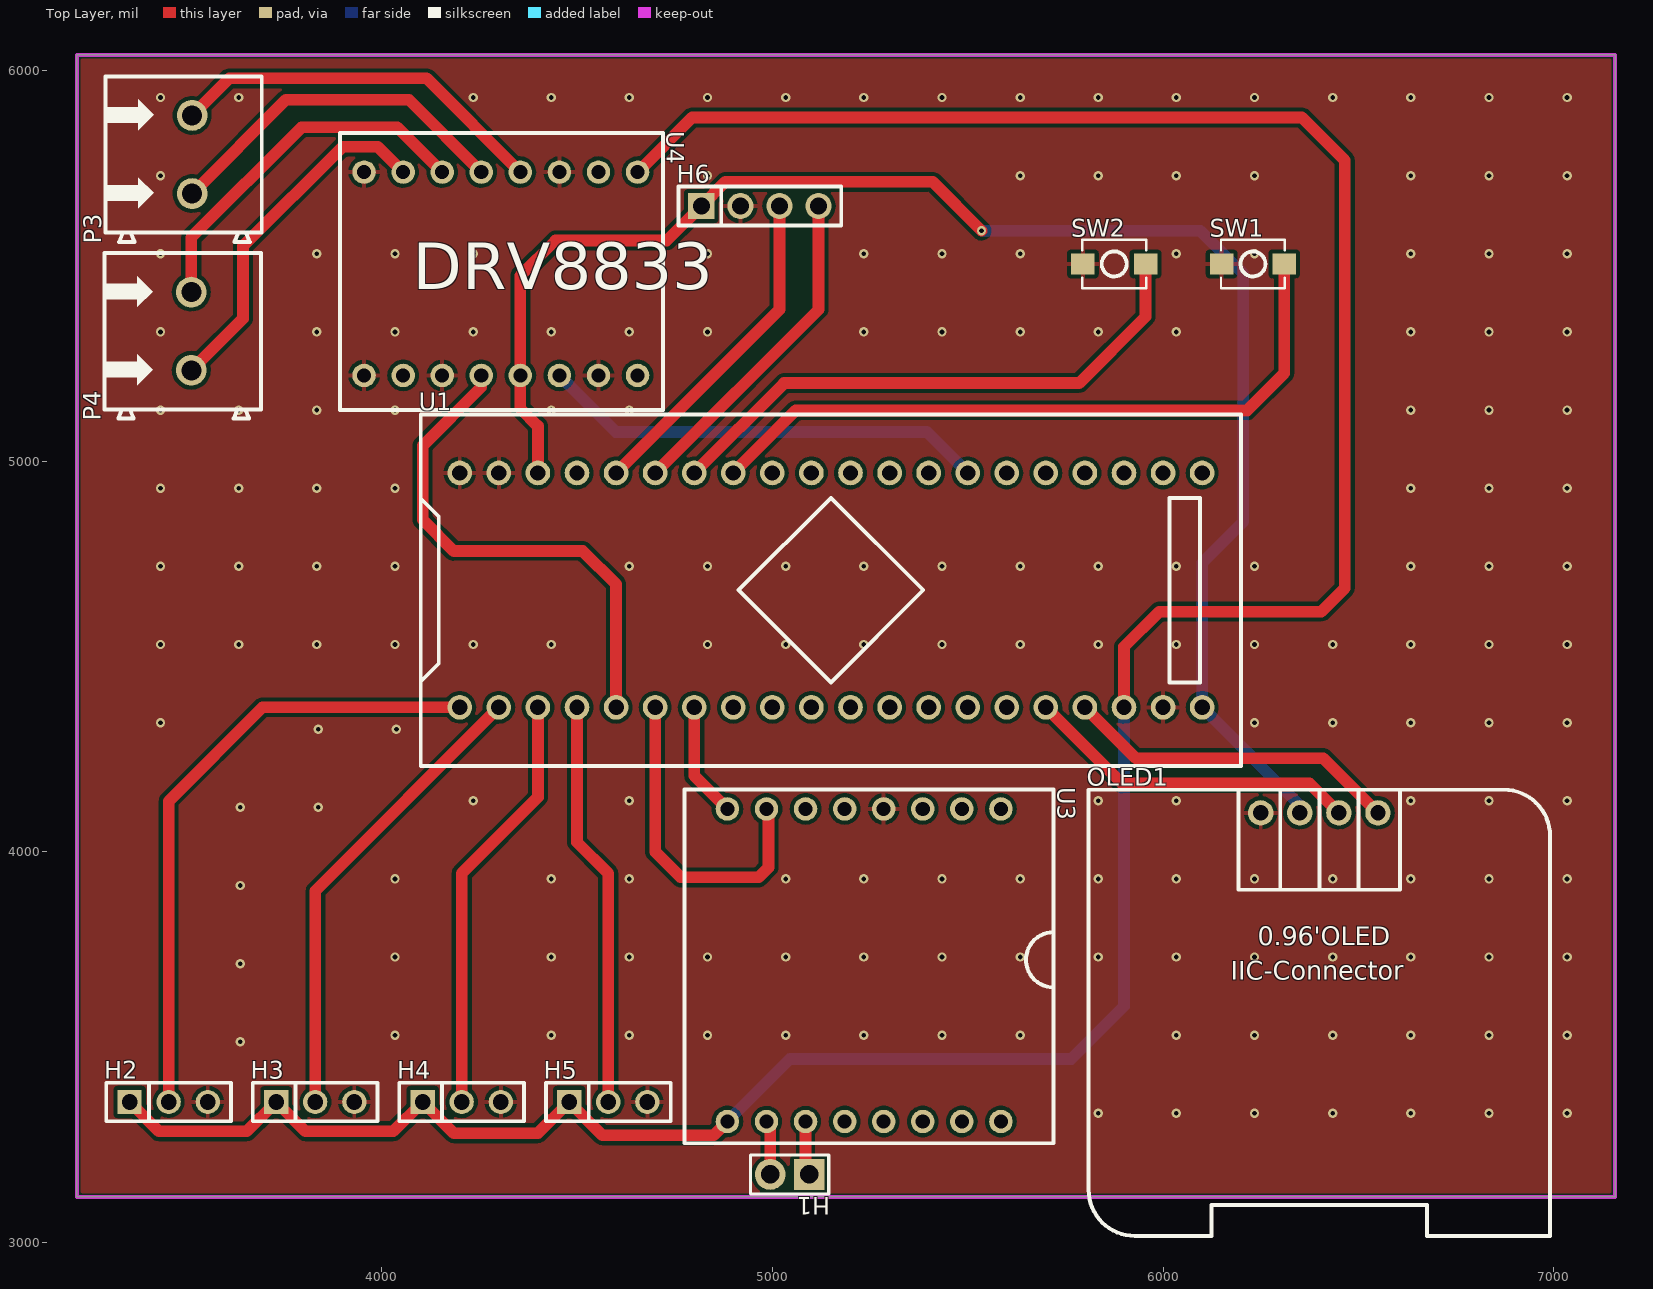
[diagram p0: Top Layer view]
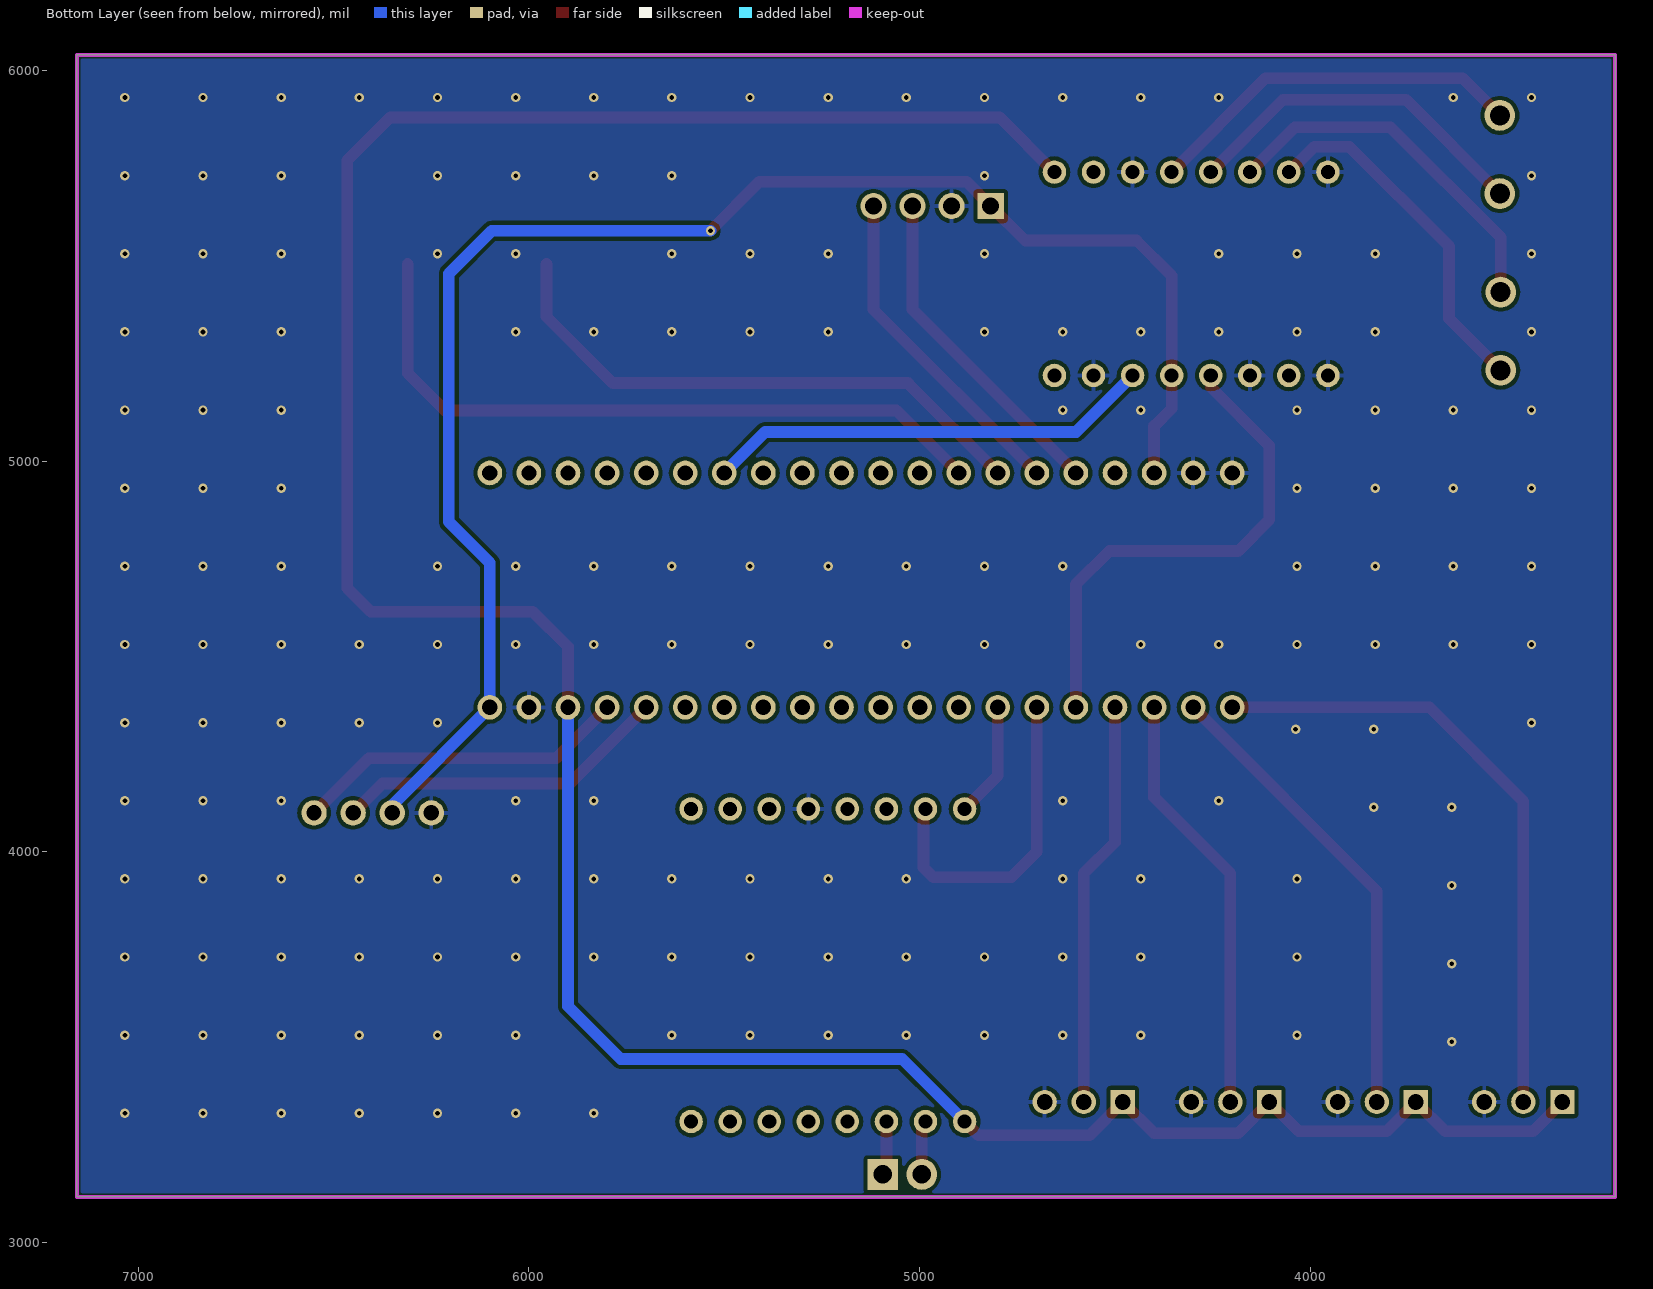
[diagram p1: Bottom Layer view, seen from below]
# Altium PCB MISC49887.pcbdoc
Units mil, origin at the board's own origin, x right, y up, seen from the top; angles counter-clockwise.
Board outline 3937.01 x 2923.15 mil, 2 copper layers (Top Layer, Bottom Layer), stack 62.206 mil thick; 14 components, 24 nets, 102 pads, 175 vias.

## Layer stack, top to bottom
Top Solder Mask Layer: solder mask 0.394, Dk 3.3
Top Layer: signal copper 1.379
Dielectric1: surface 59.449, FR4, Dk 4.5
Bottom Layer: signal copper 1.378
Bottom Solder Mask Layer: solder mask 0.394, Dk 3.3

## Board outline
3220,6040 3220,3116.85 7157.01,3116.85 7157.01,6040

## Design rules (kind name [scope] priority, off if disabled: settings)
BoardOutlineClearance copperThickness2oz_1 [All] p2 off: genericclearance=7.99 ignorepadtopadclearanceinfootprint=FALSE except(0: Arc-SplitContinuation Track-SplitContinuation SMDPad-SplitContinuation THPad-SplitContinuation Via-SplitContinuation Fill-SplitContinuation Region-SplitContinuation Poly-SplitContinuation Text-SplitContinuation Hole-SplitContinuation; 5.98: Arc-CutoutEdge SMDPad-CutoutEdge THPad-CutoutEdge Via-CutoutEdge Fill-CutoutEdge Region-CutoutEdge Text-CutoutEdge; 6.93: Hole-OutlineEdge Hole-CutoutEdge; 10: Poly-OutlineEdge Poly-CutoutEdge; 11.81: Arc-OutlineEdge Track-OutlineEdge SMDPad-OutlineEdge THPad-OutlineEdge Via-OutlineEdge Fill-OutlineEdge Region-OutlineEdge Text-OutlineEdge Track-CutoutEdge)
BoardOutlineClearance copperThickness1oz_1 [All] p4: genericclearance=4.02 ignorepadtopadclearanceinfootprint=FALSE except(0: Arc-SplitContinuation Track-SplitContinuation SMDPad-SplitContinuation THPad-SplitContinuation Via-SplitContinuation Fill-SplitContinuation Region-SplitContinuation Poly-SplitContinuation Text-SplitContinuation Hole-SplitContinuation; 6: SMDPad-CutoutEdge THPad-CutoutEdge Via-CutoutEdge Fill-CutoutEdge Region-CutoutEdge Text-CutoutEdge; 6.93: Hole-OutlineEdge Hole-CutoutEdge; 10: Poly-OutlineEdge Poly-CutoutEdge; 11.8: Arc-OutlineEdge Track-OutlineEdge SMDPad-OutlineEdge THPad-OutlineEdge Via-OutlineEdge Fill-OutlineEdge Region-OutlineEdge Text-OutlineEdge; 11.81: Arc-CutoutEdge Track-CutoutEdge)
Clearance copperThickness2oz [All] p1 off: gap=7.99 ignorepadtopadclearanceinfootprint=FALSE except(5.98: SMDPad-Track SMDPad-SMDPad THPad-Track SMDPad-THPad THPad-THPad Track-Via SMDPad-Via THPad-Via Via-Via Fill-Track Region-Track Fill-SMDPad Region-SMDPad Fill-THPad Region-THPad Fill-Via Region-Via Fill-Fill Fill-Region Region-Region Arc-Track Arc-SMDPad Arc-THPad Arc-Via Fill-Arc Region-Arc Arc-Arc Text-Track SMDPad-Text Text-THPad Text-Via Fill-Text Region-Text Arc-Text Text-Text; 6.93: Hole-Track Hole-SMDPad Hole-THPad Hole-Via Fill-Hole Region-Hole Hole-Arc Hole-Text; 10: Poly-Track Poly-SMDPad Poly-THPad Poly-Via Poly-Fill Poly-Region Poly-Poly Poly-Arc Poly-Text Poly-Hole)
Clearance copperThickness1oz [All] p3: gap=4.02 ignorepadtopadclearanceinfootprint=FALSE except(5.98: SMDPad-Track SMDPad-SMDPad THPad-Track SMDPad-THPad THPad-THPad Track-Via SMDPad-Via THPad-Via Via-Via Fill-Track Region-Track Fill-SMDPad Region-SMDPad Fill-THPad Region-THPad Fill-Via Region-Via Fill-Fill Fill-Region Region-Region; 6: Arc-Track Arc-SMDPad Arc-THPad Arc-Via Fill-Arc Region-Arc Arc-Arc Text-Track SMDPad-Text Text-THPad Text-Via Fill-Text Region-Text Arc-Text Text-Text; 6.93: Hole-Track Hole-SMDPad Hole-THPad Hole-Via Fill-Hole Region-Hole Hole-Arc Hole-Text; 10: Poly-Track Poly-SMDPad Poly-THPad Poly-Via Poly-Fill Poly-Region Poly-Poly Poly-Arc Poly-Text Poly-Hole)
DiffPairsRouting differentialPair [All] p1: maxlimit=6 minlimit=6 mostfreqgap=6 toplayer_minwidth=5 toplayer_prefwidth=10 toplayer_maxwidth=100 toplayer_mingap=6 toplayer_prefgap=6 toplayer_maxgap=6 bottomlayer_minwidth=5 bottomlayer_prefwidth=10 bottomlayer_maxwidth=100 bottomlayer_mingap=6 bottomlayer_prefgap=6 bottomlayer_maxgap=6 maxuncoupledlength=10
HoleToHoleClearance otherClearance [All] p1: gap=11.81 allowstackedmicrovias=TRUE
Length netLength [All] p1: minlimit=0 maxlimit=0
MatchedLengths netLengthTolerance [All] p1: tolerance=1000
PasteMaskExpansion pasteMaskExpansion [All] p1: expansion=0
PlaneConnect innerPlane [All] p1: planeconnectstyle=Relief reliefexpansion=20 reliefentries=4 reliefconductorwidth=10 reliefairgap=10
PolygonConnect copperRegion [(InNet('GND'))] p1: connectstyle=Relief reliefconductorwidth=10 reliefentries=4 polygonreliefangle="90 Angle" airgapwidth=10 via.connectstyle=Relief via.reliefconductorwidth=10 via.reliefentries=4 via.polygonreliefangle="90 Angle" via.airgapwidth=10
RoutingVias viaSize [All] p1: holewidth=12.01 width=24.02 viastyle="Through Hole" minholewidth=11.81 minwidth=19.68 maxholewidth=248.03 maxwidth=393.7
SolderMaskExpansion solderMaskExpansion [IsVia] p1: expansion=-1000 istentingtop=TRUE
SolderMaskExpansion solderMaskExpansion [All] p2: expansion=2 istentingtop=FALSE
Width copperThickness2oz_2 [All] p1 off: maxlimit=100 minlimit=8 preferedwidth=10
Width copperThickness1oz_2 [All] p2: maxlimit=100 minlimit=5 preferedwidth=10

## Components (designator, comment, footprint, x,y, rotation, side; value= is the part's Value field where it differs from the comment)
H1 "HX PH254-01-02-Z-L11.5 male header connector" HDR-TH_2P-P2.54-V-M 5044.44,3174.56 r180 top
H2 "" HDR-TH_3P-P2.54-V-F 3455,3360 r0 top
H3 "" HDR-TH_3P-P2.54-V-F 3830,3360 r0 top
H4 "" HDR-TH_3P-P2.54-V-F 4205,3360 r0 top
H5 "" HDR-TH_3P-P2.54-V-F 4580,3360 r0 top
H6 "" HDR-TH_4P-P2.54-V-F 4968.17,5653.05 r0 top
OLED1 "" 0.96OLED_4P 6400,4100 r0 top
P3 "WJ500V-5.08-2P" CONN-TH_2P-P5.00_WJ500V-5.08-2P 3515,5785 r90 top
P4 "WJ500V-5.08-2P" CONN-TH_2P-P5.00_WJ500V-5.08-2P 3512.81,5332.81 r90 top
SW1 "" Key_SMD_3x4x2 6230,5505 r0 top
SW2 "" Key_SMD_3x4x2 5875,5505 r0 top
U1 "STM32F103C8T6" CONN-TH_L53.3-W22.9_STM32F103C8T6-CARD 5150,4670 r0 top
U3 "" MY2490-16P 5265,3720 r270 top
U4 "" DRV8833 3705,4280 r270 top

## Footprints (in the part's own frame and the unit in brackets; to place one, negate y for a bottom-side part, rotate by r counter-clockwise, add the part's x,y. Pads: shape width x height; smd on the part's side, far side on the other; paste and mask are expansions set on the pad)
0.96OLED_4P [mm]
  round 1.65 hole 1 copper offset 0,0: 1(-3.81,-0.001) 2(-1.27,0.002) 3(1.27,0.002) 4(3.81,0.002)
  silkscreen extent -15,-27.5 15,1.5
CONN-TH_2P-P5.00_WJ500V-5.08-2P [mm]
  round 2 hole 1.3: 1(-2.54,0) 2(2.54,0)
  silkscreen extent -5.68,-4.52 5.08,5.64
CONN-TH_L53.3-W22.9_STM32F103C8T6-CARD [mm]
  round 1.6 hole 1: 1(-24.13,-7.62) 2(-21.59,-7.62) 3(-19.05,-7.62) 4(-16.51,-7.62) 5(-13.97,-7.62) 6(-11.43,-7.62) 7(-8.89,-7.62) 8(-6.35,-7.62) 9(-3.81,-7.62) 10(-1.27,-7.62) 11(1.27,-7.62) 12(3.81,-7.62) 13(6.35,-7.62) 14(8.89,-7.62) 15(11.43,-7.62) 16(13.97,-7.62) 17(16.51,-7.62) 18(19.05,-7.62) 19(21.59,-7.62) 20(24.13,-7.62) 21(24.13,7.62) 22(21.59,7.62) 23(19.05,7.62) 24(16.51,7.62) 25(13.97,7.62) 26(11.43,7.62) 27(8.89,7.62) 28(6.35,7.62) 29(3.81,7.62) 30(1.27,7.62) 31(-1.27,7.62) 32(-3.81,7.62) 33(-6.35,7.62) 34(-8.89,7.62) 35(-11.43,7.62) 36(-13.97,7.62) 37(-16.51,7.62) 38(-19.05,7.62) 39(-21.59,7.62) 40(-24.13,7.62)
  silkscreen extent -26.67,-11.43 26.67,11.43
DRV8833 [mil]
  round 60 hole 36: 1(-1460,950) 2(-1460,850) 3(-1460,750) 4(-1460,650) 5(-1460,550) 6(-1460,450) 7(-1460,350) 8(-1460,250) 9(-939.51,250) 10(-939.51,350) 11(-939.51,450) 12(-939.51,550) 13(-939.51,650) 14(-939.51,750) 15(-939.51,850) 16(-939.51,950)
  silkscreen extent -1560,188 -851,1015
HDR-TH_2P-P2.54-V-M [mm]
  rect 2x2 hole 1.2: 1(-1.27,0)
  round 2 hole 1.2: 2(1.27,0)
  silkscreen extent -2.54,-1.27 2.54,1.27
HDR-TH_3P-P2.54-V-F [mil]
  rect 62x62 hole 40.16: 1(-100,0)
  round 62 hole 40.16: 2(0,0) 3(100,0)
  silkscreen extent -160,-49 160,49
HDR-TH_4P-P2.54-V-F [mm]
  rect 1.7x1.7 hole 1.1: 1(-3.81,0)
  round 1.7 hole 1.1: 2(-1.27,0) 3(1.27,0) 4(3.81,0)
  silkscreen extent -5.29,-1.27 5.29,1.27
Key_SMD_3x4x2 [mm]
  rect 1.53x1.36 smd paste+0 mask+0.051: 1(-2.035,0) 2(2.035,0)
  silkscreen extent -2.08,-1.58 2.08,1.58
MY2490-16P [mil]
  round 60 hole 36: 1(-390,320) 2(-390,220) 3(-390,120) 4(-390,20) 5(-390,-80) 6(-390,-180) 7(-390,-280) 8(-390,-380) 9(410,-380) 10(410,-280) 11(410,-180) 12(410,-80) 13(410,20) 14(410,120) 15(410,220) 16(410,320)
  silkscreen extent -440,-490 466,455

## Via types
v1: diameter 24.02, hole 12, Top Layer to Bottom Layer, 175 vias

## Nets (pads, with @x,y where several pads share a name; then routed paths per layer and width w, separated by ;. In a path a pad name is that pad's centre, name@x,y a point inside that pad or via, vN(x,y) a via of type N, cw(c..) or ccw(c..) an arc to the next point about the centre after c; other vN are vias at no path point)
$1N4770: P3.2 U4.4 | length 978.8
  Top Layer w30: P3.2 3610,5980 4115,5980 U4.4
$1N4771: P3.1 U4.5 | length 916
  Top Layer w30: P3.1 3755,5925 4070,5925 U4.5
$1N4772: P4.2 U4.6 | length 946.7
  Top Layer w30: P4.2 3512.81,5572.81 3795,5855 4040,5855 U4.6
$1N4773: P4.1 U4.7 | length 914.5
  Top Layer w30: P4.1 3645,5365 3645,5550 3900,5805 3990,5805 U4.7
+3.3V: H6.1 OLED1.2 U1.20 U1.38 U4.13 | length 4097.4
  Top Layer w30: U1.38 4400,5090 4355,5135 U4.13 4355,5475 4445,5565 4730,5565 4818.11,5653.11 4880,5715 5410.28,5715 v1(5535.28,5590)
  Bottom Layer w30: v1(5535.28,5590) 6095,5590 6205,5480 6205,4845 6100,4740 U1.20 6350,4120 OLED1.2@6350,4100.05
+5V: H2.1 H3.1 H4.1 H5.1 U1.18 U3.9 U4.1 | length 7463.1
  Top Layer w30: H2.1 3430,3285 3655,3285 H3.1 3805,3285 4030,3285 H4.1 4185,3280 4400,3280 H5.1 4565,3275 4850,3275 U3.9 ; U4.1 4795,5880 6355,5880 6465,5770 6465,4675 6405,4615 5990,4615 5900,4525 U1.18
  Bottom Layer w30: U3.9 5045,3470 5765,3470 5900,3605 U1.18
GND: H2.3 H3.3 H4.3 H5.3 H6.2 OLED1.1 SW1.1 SW2.1 U1.19 U1.39 U1.40 U3.4 U4.3 U4.8 U4.9 U4.11 U4.15
  other v1: 5834.1,3330.95 6034.1,3330.95 6234.1,3330.95 6434.1,3330.95 6634.1,3330.95 6834.1,3330.95 7034.1,3330.95 3637.88,3514.1 4034.1,3530.95 4434.1,3530.95 4634.1,3530.95 4834.1,3530.95 5034.1,3530.95 5234.1,3530.95 5434.1,3530.95 5634.1,3530.95 6034.1,3530.95 6234.1,3530.95 6434.1,3530.95 6634.1,3530.95 6834.1,3530.95 7034.1,3530.95 3637.88,3714.1 4034.1,3730.95 4434.1,3730.95 4634.1,3730.95 4834.1,3730.95 5034.1,3730.95 5234.1,3730.95 5434.1,3730.95 5634.1,3730.95 5834.1,3730.95 6034.1,3730.95 6234.1,3730.95 6434.1,3730.95 6634.1,3730.95 6834.1,3730.95 7034.1,3730.95 3637.88,3914.1 4034.1,3930.95 4434.1,3930.95 4634.1,3930.95 5034.1,3930.95 5234.1,3930.95 5434.1,3930.95 5634.1,3930.95 5834.1,3930.95 6034.1,3930.95 6234.1,3930.95 6434.1,3930.95 6634.1,3930.95 6834.1,3930.95 7034.1,3930.95 3637.88,4114.1 3837.88,4114.1 4234.1,4130.95 4634.1,4130.95 5834.1,4130.95 6034.1,4130.95 6634.1,4130.95 6834.1,4130.95 7034.1,4130.95 3837.88,4314.1 4037.88,4314.1 3434.1,4330.95 6234.1,4330.95 6434.1,4330.95 6634.1,4330.95 6834.1,4330.95 7034.1,4330.95 3434.1,4530.95 3634.1,4530.95 3834.1,4530.95 4034.1,4530.95 4234.1,4530.95 4434.1,4530.95 4834.1,4530.95 5034.1,4530.95 5234.1,4530.95 5434.1,4530.95 5634.1,4530.95 5834.1,4530.95 6034.1,4530.95 6234.1,4530.95 6434.1,4530.95 6634.1,4530.95 6834.1,4530.95 7034.1,4530.95 3434.1,4730.95 3634.1,4730.95 3834.1,4730.95 4034.1,4730.95 4634.1,4730.95 4834.1,4730.95 5034.1,4730.95 5234.1,4730.95 5434.1,4730.95 5634.1,4730.95 5834.1,4730.95 6034.1,4730.95 6234.1,4730.95 6634.1,4730.95 6834.1,4730.95 7034.1,4730.95 3434.1,4930.95 3634.1,4930.95 3834.1,4930.95 4034.1,4930.95 6634.1,4930.95 6834.1,4930.95 7034.1,4930.95 3434.1,5130.95 3634.1,5130.95 3834.1,5130.95 4034.1,5130.95 4434.1,5130.95 4634.1,5130.95 6634.1,5130.95 6834.1,5130.95 7034.1,5130.95 3434.1,5330.95 3834.1,5330.95 4034.1,5330.95 4234.1,5330.95 4434.1,5330.95 4634.1,5330.95 4834.1,5330.95 5234.1,5330.95 5434.1,5330.95 5634.1,5330.95 5834.1,5330.95 6034.1,5330.95 6634.1,5330.95 6834.1,5330.95 7034.1,5330.95 3434.1,5530.95 3834.1,5530.95 4034.1,5530.95 4234.1,5530.95 4834.1,5530.95 5234.1,5530.95 5434.1,5530.95 5634.1,5530.95 6034.1,5530.95 6234.1,5530.95 6634.1,5530.95 6834.1,5530.95 7034.1,5530.95 3434.1,5730.95 4834.1,5730.95 5634.1,5730.95 5834.1,5730.95 6034.1,5730.95 6234.1,5730.95 6634.1,5730.95 6834.1,5730.95 7034.1,5730.95 3434.1,5930.95 3634.1,5930.95 4234.1,5930.95 4434.1,5930.95 4634.1,5930.95 4834.1,5930.95 5034.1,5930.95 5234.1,5930.95 5434.1,5930.95 5634.1,5930.95 5834.1,5930.95 6034.1,5930.95 6234.1,5930.95 6434.1,5930.95 6634.1,5930.95 6834.1,5930.95 7034.1,5930.95
PA0: U1.25
PA2: U1.27 U4.14 | length 1148.4
  Bottom Layer w30: U4.14 4599.51,5075 5395,5075 U1.27
PA8: U1.5 U4.12 | length 1310
  Top Layer w30: U4.12 4255,5190 4105,5040 4105,4850 4185,4770 4515,4770 4600,4685 U1.5
PA9: U1.6 U3.7 | length 849.4
  Top Layer w30: U1.6 4700,4000 4765,3935 4965,3935 4990,3960 4990,4105 U3.7
PA10: U1.7 U3.8 | length 295.2
  Top Layer w30: U1.7 4800,4195 U3.8
PB0: SW1.2 U1.33 | length 1795.7
  Top Layer w30: U1.33 5060,5130 6215,5130 6310.12,5225.12 SW1.2
PB1: SW2.2 U1.34 | length 1455.7
  Top Layer w30: U1.34 5030,5200 5785,5200 5955.12,5370.12 SW2.2
PB8: OLED1.3 U1.16 | length 861.8
  Top Layer w30: U1.16 5895,4175 6375.05,4175 OLED1.3@6450,4100.05
PB9: OLED1.4 U1.17 | length 861.8
  Top Layer w30: U1.17 5930,4240 6410.05,4240 OLED1.4@6550,4100.05
PB10: H6.4 U1.35 | length 856.3
  Top Layer w30: U1.35 5118.17,5388.17 H6.4
PB11: H6.3 U1.36 | length 856.3
  Top Layer w30: U1.36 5018.17,5388.17 H6.3
PB12: H2.2 U1.1 | length 1614.4
  Top Layer w30: H2.2 3455,4130 3695,4370 U1.1
PB13: H3.2 U1.2 | length 1204.7
  Top Layer w30: H3.2 3830,3900 U1.2
PB14: H4.2 U1.3 | length 1090.8
  Top Layer w30: H4.2 4205,3945 4400,4140 U1.3
PB15: H5.2 U1.4 | length 1043.1
  Top Layer w30: U1.4 4500,4025 4580,3945 H5.2
SPK1: H1.1 U3.11 | length 139.4
  Top Layer w30: U3.11 5085,3184 H1.1
SPK2: H1.2 U3.10 | length 139.4
  Top Layer w30: U3.10 4994.44,3300.56 H1.2
pads on no net: U1.8 U1.9 U1.10 U1.11 U1.12 U1.13 U1.14 U1.15 U1.21 U1.22 U1.23 U1.24 U1.26 U1.28 U1.29 U1.30 U1.31 U1.32 U1.37 U3.1 U3.2 U3.3 U3.5 U3.6 U3.12 U3.13 U3.14 U3.15 U3.16 U4.2 U4.10 U4.16

## Polygon pours and split planes (outlines as drawn)
GND on Top Layer (solid, remove dead copper, pour order 0): 3075,6345 3075,3040 7350,3040 7350,6345
GND on Bottom Layer (solid, remove dead copper, pour order 2): 3000,6190 3000,3000 7390,3000 7390,6190

## Keep-outs
Board Outline Layer:
  the board outline again, w10